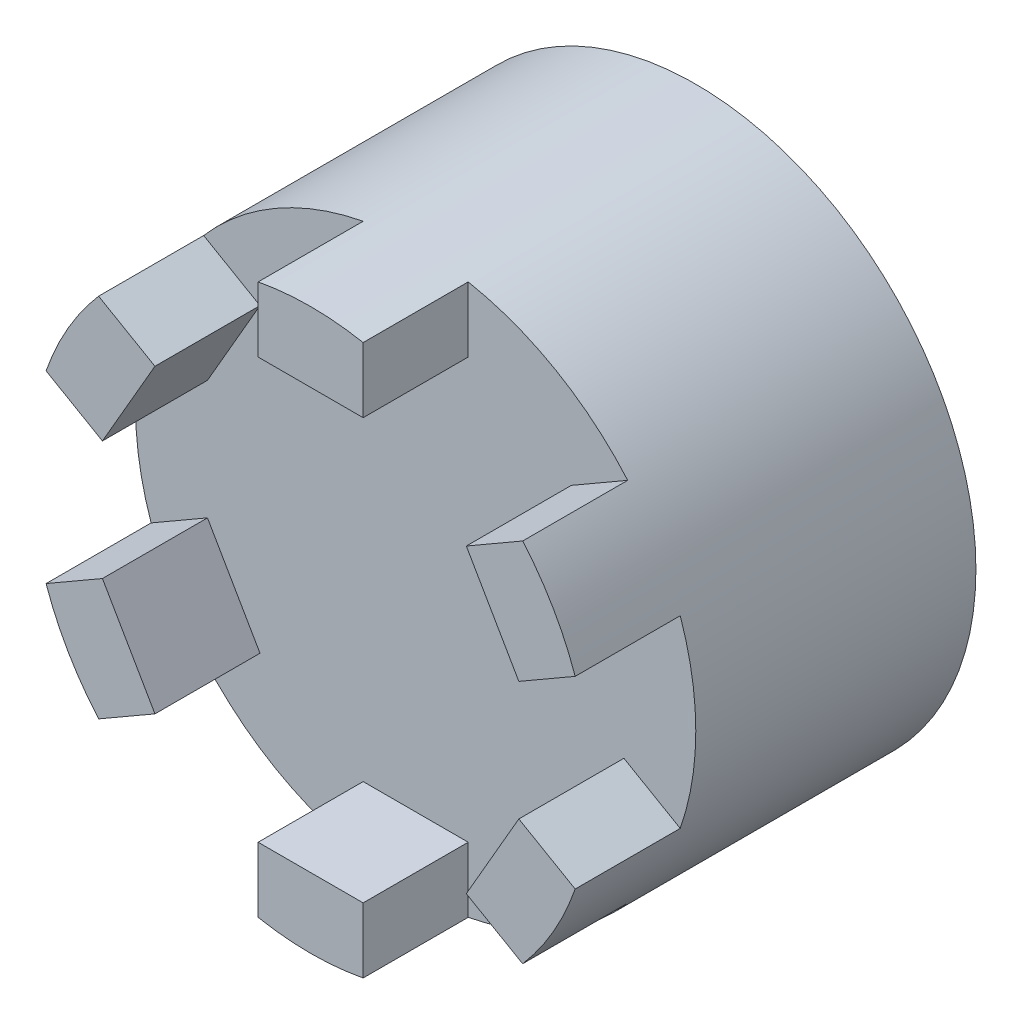
from build123d import *

# Parameters (mm, degrees)
SKETCH_2_R          = 40
EXTRUDE_1_DEPTH     = 40
SKETCH_1_R          = 16.5
CUT_EXTRUDE_1_DEPTH = 30
EXTRUDE_2_DEPTH     = 15
SKETCH_4_W          = 12
SKETCH_4_H          = 7.528633981
CUT_EXTRUDE_2_DEPTH = 30


with BuildPart() as part:
    # 草图2 → 凸台-拉伸1 (new body)
    with BuildSketch(Plane.XY):
        Circle(SKETCH_2_R)
    extrude(amount=EXTRUDE_1_DEPTH)

    # 草图1 → 切除-拉伸1 (cut)
    with BuildSketch(Plane.XY):
        Circle(SKETCH_1_R)
    extrude(amount=CUT_EXTRUDE_1_DEPTH, mode=Mode.SUBTRACT)

    # 草图3 → 凸台-拉伸2 (add)
    with BuildSketch(Plane.XY.offset(40)):
        with BuildLine():
            Line((22.230762114, 21.495190528), (29.730762114, 8.504809472))
            Line((29.730762114, 8.504809472), (37.776643972, 13.150101528))
            ThreePointArc((37.776643972, 13.150101528), (34.641016151, 20), (30.276643972, 26.140482585))
            Line((30.276643972, 26.140482585), (22.230762114, 21.495190528))
        make_face()
        with BuildLine():
            Line((-7.5, 39.290584114), (-7.5, 30))
            Line((-7.5, 30), (7.5, 30))
            Line((7.5, 30), (7.5, 39.290584114))
            ThreePointArc((7.5, 39.290584114), (0, 40), (-7.5, 39.290584114))
        make_face()
        with BuildLine():
            Line((29.730762114, -8.504809472), (22.230762114, -21.495190528))
            Line((22.230762114, -21.495190528), (30.276643972, -26.140482585))
            ThreePointArc((30.276643972, -26.140482585), (34.641016151, -20), (37.776643972, -13.150101528))
            Line((37.776643972, -13.150101528), (29.730762114, -8.504809472))
        make_face()
        with BuildLine():
            Line((7.5, -30), (-7.5, -30))
            Line((-7.5, -30), (-7.5, -39.290584114))
            ThreePointArc((-7.5, -39.290584114), (0, -40), (7.5, -39.290584114))
            Line((7.5, -39.290584114), (7.5, -30))
        make_face()
        with BuildLine():
            Line((-22.230762114, -21.495190528), (-29.730762114, -8.504809472))
            Line((-29.730762114, -8.504809472), (-37.776643972, -13.150101528))
            ThreePointArc((-37.776643972, -13.150101528), (-34.641016151, -20), (-30.276643972, -26.140482585))
            Line((-30.276643972, -26.140482585), (-22.230762114, -21.495190528))
        make_face()
        with BuildLine():
            Line((-29.730762114, 8.504809472), (-22.230762114, 21.495190528))
            Line((-22.230762114, 21.495190528), (-30.276643972, 26.140482585))
            ThreePointArc((-30.276643972, 26.140482585), (-34.641016151, 20), (-37.776643972, 13.150101528))
            Line((-37.776643972, 13.150101528), (-29.730762114, 8.504809472))
        make_face()
    extrude(amount=EXTRUDE_2_DEPTH)

    # 草图4 → 切除-拉伸2 (cut)
    with BuildSketch(Plane(origin=(0, 0, 0), x_dir=(-1, 0, 0), z_dir=(0, 0, -1))):
        with Locations((0, 15.23568301)):
            Rectangle(SKETCH_4_W, SKETCH_4_H)
    extrude(amount=-CUT_EXTRUDE_2_DEPTH, mode=Mode.SUBTRACT)


solid = part.part
